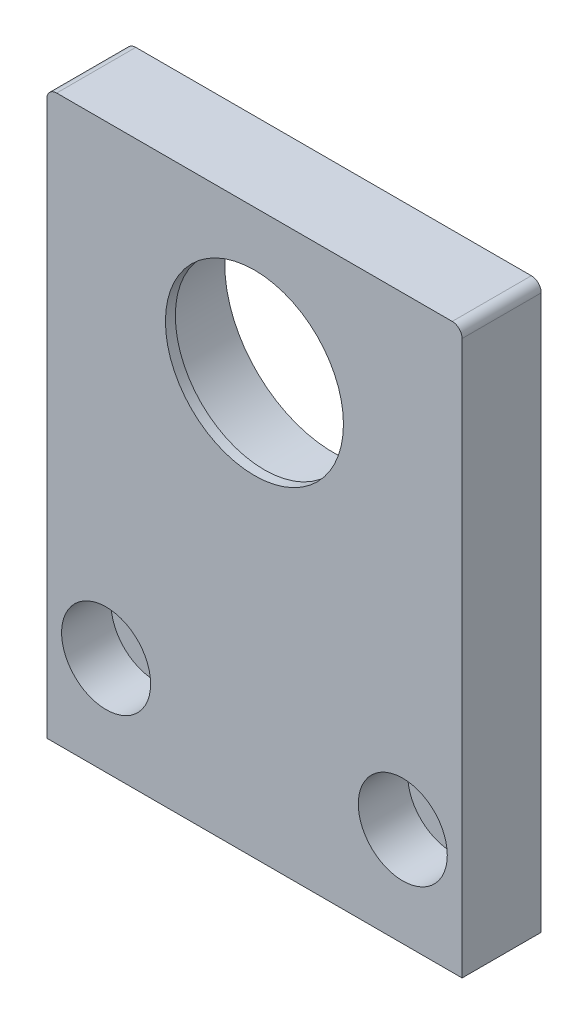
from build123d import *

# Parameters (mm, degrees)
SKETCH1_R           = 9
SKETCH1_R_2         = 2.5
BOSS_EXTRUDE1_DEPTH = 8
SKETCH2_R           = 4.5
CUT_EXTRUDE1_DEPTH  = 5
SKETCH3_R           = 11
CUT_EXTRUDE2_DEPTH  = 7


with BuildPart() as part:
    # Sketch1 → Boss-Extrude1 (new body)
    with BuildSketch(Plane.XY):
        with BuildLine():
            Line((-20, 28.5), (20, 28.5))
            ThreePointArc((20, 28.5), (20.707106781, 28.207106781), (21, 27.5))
            Line((21, 27.5), (21, -28.5))
            Line((21, -28.5), (-21, -28.5))
            Line((-21, -28.5), (-21, 27.5))
            ThreePointArc((-21, 27.5), (-20.707106781, 28.207106781), (-20, 28.5))
        make_face()
        with Locations((0, 14)):
            Circle(SKETCH1_R, mode=Mode.SUBTRACT)
        with Locations((-15, -18.5)):
            Circle(SKETCH1_R_2, mode=Mode.SUBTRACT)
        with Locations((15, -18.5)):
            Circle(SKETCH1_R_2, mode=Mode.SUBTRACT)
    extrude(amount=BOSS_EXTRUDE1_DEPTH)

    # Sketch2 → Cut-Extrude1 (cut)
    with BuildSketch(Plane.XY.offset(8)):
        with Locations((-15, -18.5)):
            Circle(SKETCH2_R)
        with Locations((15, -18.5)):
            Circle(SKETCH2_R)
    extrude(amount=-CUT_EXTRUDE1_DEPTH, mode=Mode.SUBTRACT)

    # Sketch3 → Cut-Extrude2 (cut)
    with BuildSketch(Plane(origin=(0, 0, 0), x_dir=(-1, 0, 0), z_dir=(0, 0, -1))):
        with Locations((0, 14)):
            Circle(SKETCH3_R)
    extrude(amount=-CUT_EXTRUDE2_DEPTH, mode=Mode.SUBTRACT)


solid = part.part
